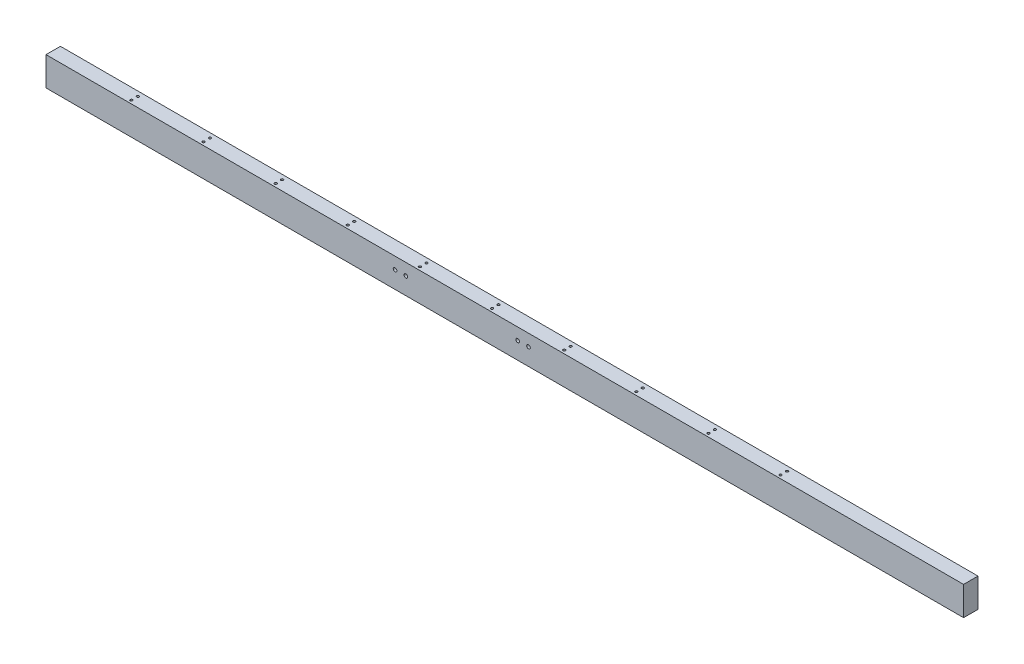
SolidWorks part; units mm, degrees
ref_plane "前视基准面" through (0, 0, 0) normal (0, 0, 1) x (1, 0, 0)
ref_plane "上视基准面" through (0, 0, 0) normal (0, 1, 0) x (1, 0, 0)
ref_plane "右视基准面" through (0, 0, 0) normal (1, 0, 0) x (0, 0, -1)
sketch "草图1" plane through (0, 0, 0) normal (0, 0, 1) x (1, 0, 0)
  line L1 (0, 0) -> (2544, 0)
  line L2 (0, 0) -> (0, -80)
  line L3 (0, -80) -> (2544, -80)
  line L4 (2544, 0) -> (2544, -80)
  dimension "D1" = 80
  dimension "D2" = 2544
extrude "凸台-拉伸1" add sketch "草图1" along normal blind 40
sketch "草图2" plane through (0, 0, 0) normal (0, 1, 0) x (1, 0, 0)
  circle A4 centre (227.7284, -13) radius 3.3355
  circle A5 centre (227.7284, -31) radius 3.3
extrude "切除-拉伸1" cut sketch "草图2" against normal blind 40
pattern_linear "阵列(线性)1" count 10 spacing 200 along (1, 0, 0) of "切除-拉伸1"
sketch "草图3" plane through (0, -80, 0) normal (0, -1, 0) x (1, 0, 0)
  circle A4 centre (458, 23.1) radius 4.5
  circle A5 centre (581, 23.1) radius 4.5
  circle A6 centre (1958, 23.1) radius 4.5
  circle A7 centre (2081, 23.1) radius 4.5
extrude "切除-拉伸2" cut sketch "草图3" against normal blind 40
sketch "草图4" plane through (0, 0, 40) normal (0, 0, 1) x (1, 0, 0)
  circle A2 centre (1337.7371, -32.6841) radius 5
  circle A3 centre (1307.7371, -32.6841) radius 5
  circle A6 centre (997.7371, -32.6841) radius 5
  circle A7 centre (967.7371, -32.6841) radius 5
extrude "切除-拉伸3" cut sketch "草图4" against normal blind 20
sketch "草图5" plane through (0, 0, 0) normal (0, 0, -1) x (-1, 0, 0)
  circle A2 centre (-1265.2371, -26) radius 7.5
  circle A3 centre (-1040.2371, -26) radius 7.5
extrude "切除-拉伸4" cut sketch "草图5" against normal blind 15
